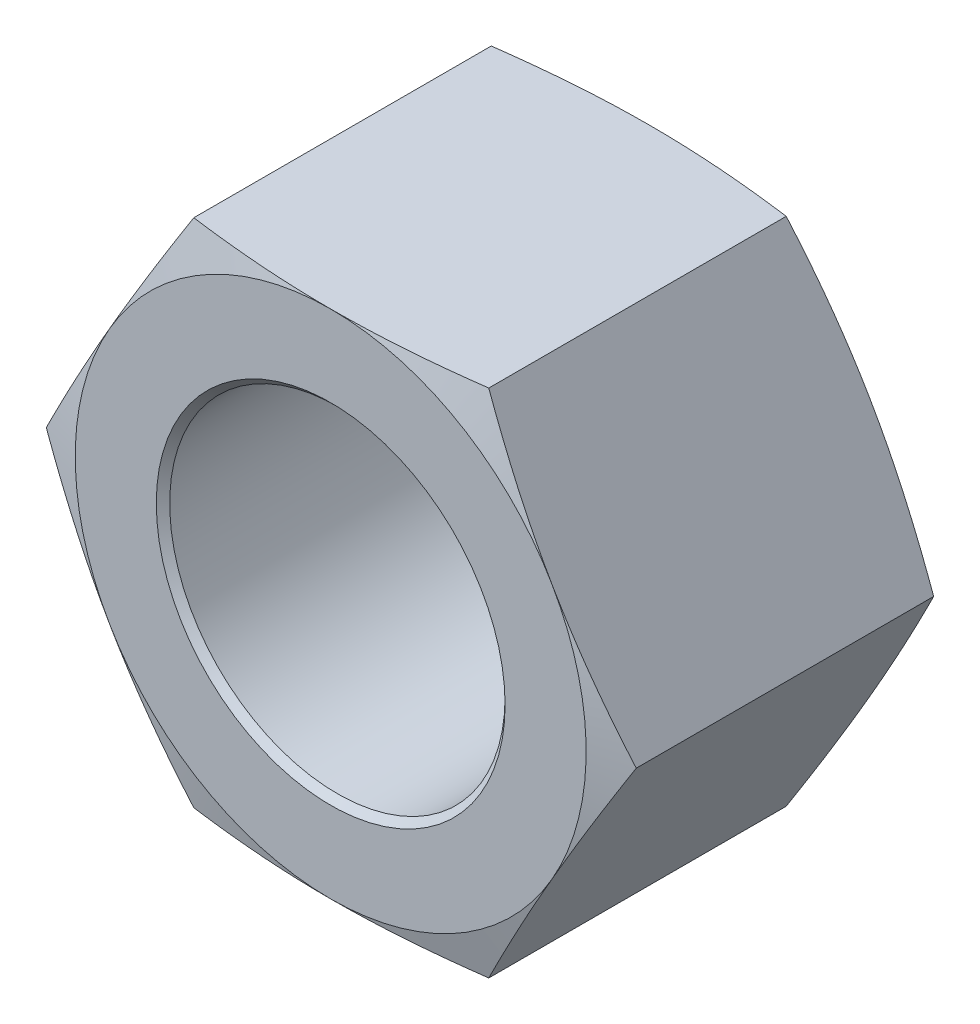
from build123d import *

# Parameters (mm, degrees)
SKETCH1_R          = 5
BOSS_EXTRUDE_DEPTH = 9.5
SKETCH2_OUTSIDE_W  = 308.252
SKETCH2_OUTSIDE_H  = 305.896
SKETCH2_OUTSIDE_R  = 7.616693426
CUT_EXTRUDE1_DEPTH = 38
CUT_EXTRUDE1_DRAFT = -75
SKETCH3_OUTSIDE_W  = 308.252
SKETCH3_OUTSIDE_H  = 305.896
SKETCH3_OUTSIDE_R  = 7.616693426
CUT_EXTRUDE2_DEPTH = 38
CUT_EXTRUDE2_DRAFT = -75
CHAMFER1_SIZE      = 0.2


with BuildPart() as part:
    # Sketch1 → Boss-Extrude (new body)
    with BuildSketch(Plane.XY):
        Polygon((4.3975, 7.616693426), (-4.3975, 7.616693426), (-8.795, 0), (-4.3975, -7.616693426), (4.3975, -7.616693426), (8.795, 0), align=None)
        Circle(SKETCH1_R, mode=Mode.SUBTRACT)
    extrude(amount=BOSS_EXTRUDE_DEPTH)


with BuildPart() as cut_extrude1_tool:
    # Sketch2 outside → Cut-Extrude1 (with draft: the straight prism first)
    with BuildSketch(Plane(origin=(0, 0, 0), x_dir=(-1, 0, 0), z_dir=(0, 0, -1))):
        Rectangle(SKETCH2_OUTSIDE_W, SKETCH2_OUTSIDE_H)
        Circle(SKETCH2_OUTSIDE_R, mode=Mode.SUBTRACT)
    extrude(amount=-CUT_EXTRUDE1_DEPTH)
    # Cut-Extrude1: the draft: its side faces are tilted about the plane it starts from
    cut_extrude1_sides = [cut_extrude1_tool.faces().sort_by_distance(p)[0] for p in [
        (0, -152.948, 19),
        (-154.126, 0, 19),
        (0, 152.948, 19),
        (154.126, 0, 19),
        (7.616693426, 0, 19),
    ]]
    draft(cut_extrude1_sides, Plane(origin=(0, 0, 0), x_dir=(-1, 0, 0), z_dir=(0, 0, -1)), CUT_EXTRUDE1_DRAFT)


with BuildPart() as part_1:
    add(part.part)

    # Cut-Extrude1: cut by cut_extrude1_tool
    add(cut_extrude1_tool.part, mode=Mode.SUBTRACT)


with BuildPart() as cut_extrude2_tool:
    # Sketch3 outside → Cut-Extrude2 (with draft: the straight prism first)
    with BuildSketch(Plane.XY.offset(9.5)):
        Rectangle(SKETCH3_OUTSIDE_W, SKETCH3_OUTSIDE_H)
        Circle(SKETCH3_OUTSIDE_R, mode=Mode.SUBTRACT)
    extrude(amount=-CUT_EXTRUDE2_DEPTH)
    # Cut-Extrude2: the draft: its side faces are tilted about the plane it starts from
    cut_extrude2_sides = [cut_extrude2_tool.faces().sort_by_distance(p)[0] for p in [
        (0, -152.948, -9.5),
        (154.126, 0, -9.5),
        (0, 152.948, -9.5),
        (-154.126, 0, -9.5),
        (-7.616693426, 0, -9.5),
    ]]
    draft(cut_extrude2_sides, Plane.XY.offset(9.5), CUT_EXTRUDE2_DRAFT)


with BuildPart() as part_2:
    add(part_1.part)

    # Cut-Extrude2: cut by cut_extrude2_tool
    add(cut_extrude2_tool.part, mode=Mode.SUBTRACT)

    # Chamfer1
    chamfer1_edges = [part_2.edges().sort_by_distance(p)[0] for p in [
        (-5, 0, 0),
        (-5, 0, 9.5),
    ]]
    chamfer(chamfer1_edges, length=CHAMFER1_SIZE)


solid = part_2.part
